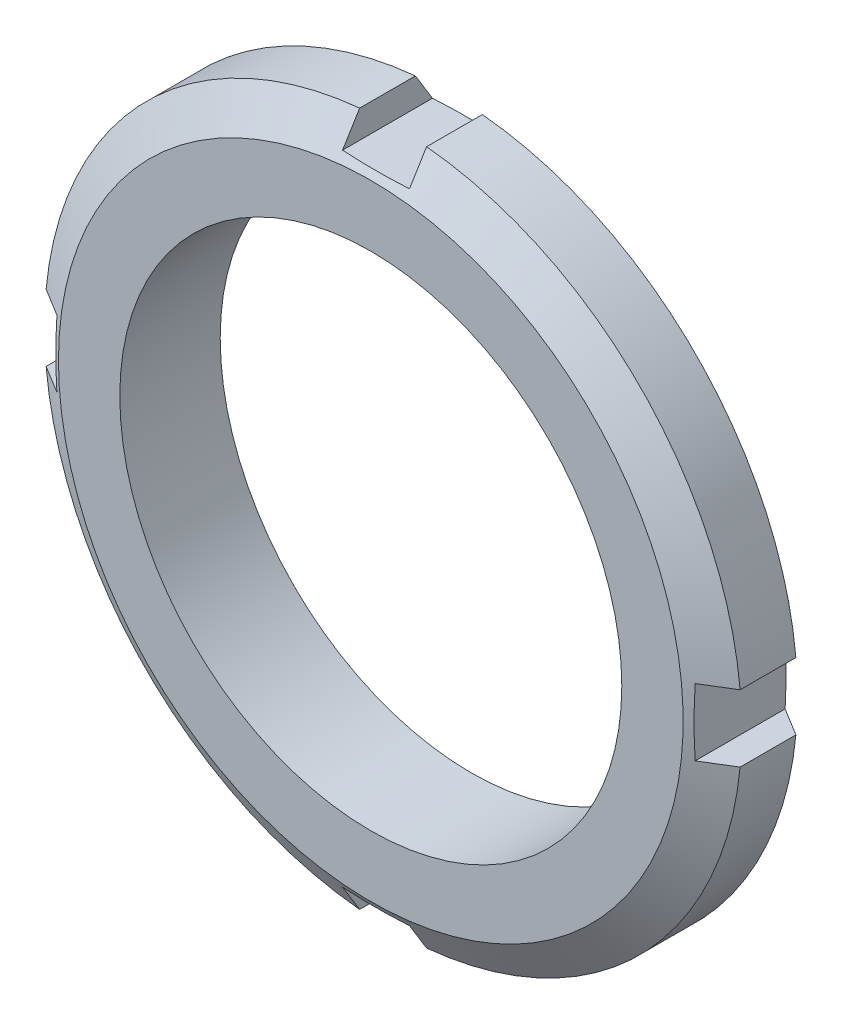
from build123d import *

# Parameters (mm, degrees)
SKETCH_1_R          = 62.5
SKETCH_1_R_2        = 45
EXTRUDE_1_DEPTH     = 18
CUT_EXTRUDE_1_DEPTH = 18


with BuildPart() as part:
    # 草图1 → 凸台-拉伸1 (new body)
    with BuildSketch(Plane.XY):
        Circle(SKETCH_1_R)
        Circle(SKETCH_1_R_2, mode=Mode.SUBTRACT)
    extrude(amount=EXTRUDE_1_DEPTH)

    # 草图2 → 切除-旋转1 (revolve, cut)
    with BuildSketch(Plane(origin=(0, 0, 0), x_dir=(1, 0, 0), z_dir=(0, 1, 0)), mode=Mode.PRIVATE) as cut_revolve_1_sk:
        Polygon((62.5, -4), (62.5, 0), (56, 0), align=None)
        Polygon((62.5, -14), (62.5, -18), (56, -18), align=None)
    revolve(cut_revolve_1_sk.sketch.rotate(Axis((0, 0, -32.669833972), (0, 0, 1)), 180), axis=Axis((0, 0, -32.669833972), (0, 0, 1)), mode=Mode.SUBTRACT)

    # 草图3 → 切除-拉伸1 (cut)
    with BuildSketch(Plane(origin=(0, 0, 0), x_dir=(-1, 0, 0), z_dir=(0, 0, -1))):
        with BuildLine():
            Line((-6, 62.211333373), (-6, 57.211333373))
            Line((-6, 57.211333373), (6, 57.211333373))
            Line((6, 57.211333373), (6, 62.211333373))
            ThreePointArc((6, 62.211333373), (0, 62.5), (-6, 62.211333373))
        make_face()
        with BuildLine():
            Line((62.211333373, 6), (57.211333373, 6))
            Line((57.211333373, 6), (57.211333373, -6))
            Line((57.211333373, -6), (62.211333373, -6))
            ThreePointArc((62.211333373, -6), (62.5, 0), (62.211333373, 6))
        make_face()
        with BuildLine():
            Line((6, -62.211333373), (6, -57.211333373))
            Line((6, -57.211333373), (-6, -57.211333373))
            Line((-6, -57.211333373), (-6, -62.211333373))
            ThreePointArc((-6, -62.211333373), (0, -62.5), (6, -62.211333373))
        make_face()
        with BuildLine():
            Line((-62.211333373, -6), (-57.211333373, -6))
            Line((-57.211333373, -6), (-57.211333373, 6))
            Line((-57.211333373, 6), (-62.211333373, 6))
            ThreePointArc((-62.211333373, 6), (-62.5, 0), (-62.211333373, -6))
        make_face()
    extrude(amount=-CUT_EXTRUDE_1_DEPTH, mode=Mode.SUBTRACT)


solid = part.part
